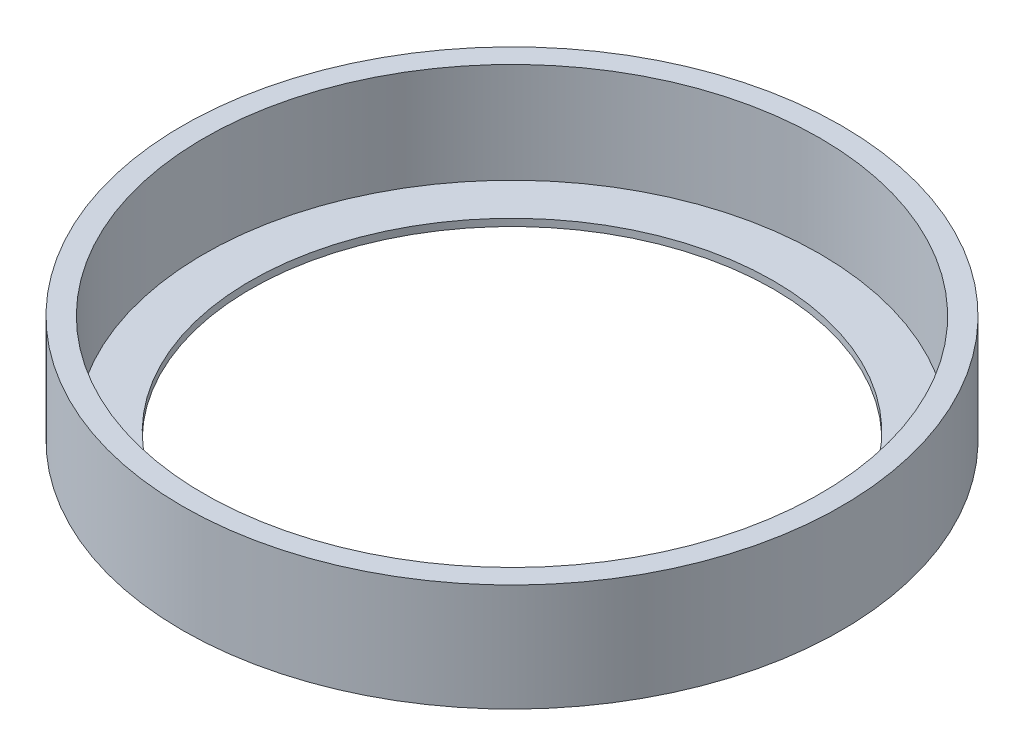
from build123d import *


with BuildPart() as part:
    # 草图1 → 旋转1 (revolve)
    with BuildSketch(Plane.XY, mode=Mode.PRIVATE) as revolve_1_sk:
        Polygon((-46, 15), (-46, 0), (-36.5, 0), (-36.5, 1), (-43, 1), (-43, 15), align=None)
    revolve(revolve_1_sk.sketch.rotate(Axis((0, 0, 0), (0, 1, 0)), 270), axis=Axis((0, 0, 0), (0, 1, 0)))


solid = part.part
